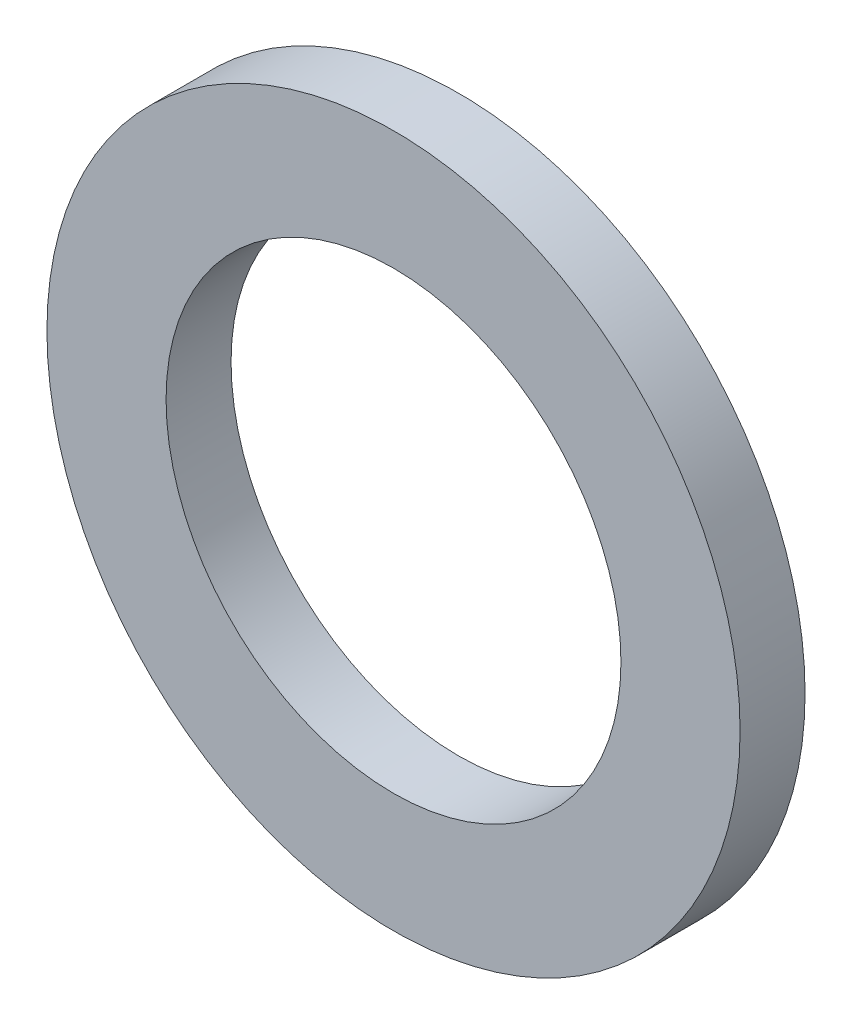
from build123d import *

# Parameters (mm, degrees)
SKETCH_246_R    = 8
SKETCH_246_R_2  = 5.25
EXTRUDE_1_DEPTH = 1.5


with BuildPart() as part:
    # Sketch 246 → 拉伸1 (new body)
    with BuildSketch(Plane.XY):
        Circle(SKETCH_246_R)
        Circle(SKETCH_246_R_2, mode=Mode.SUBTRACT)
    extrude(amount=EXTRUDE_1_DEPTH)


solid = part.part
